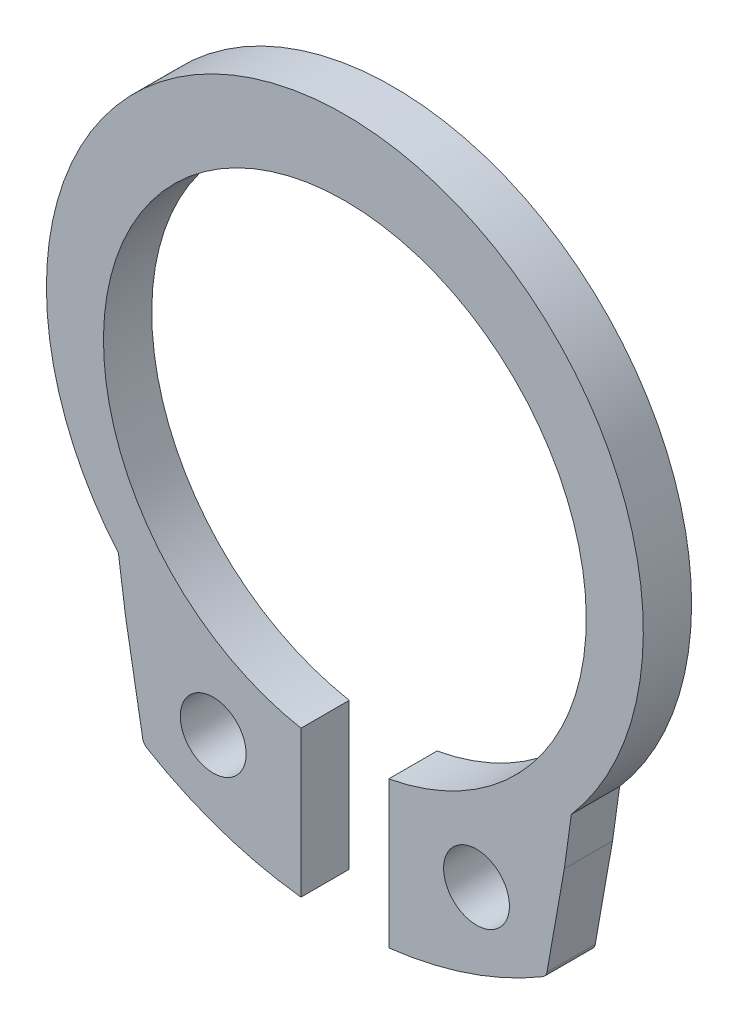
from build123d import *

# Parameters (mm, degrees)
SKETCH1_R           = 0.75
BOSS_EXTRUDE1_DEPTH = 1.1


with BuildPart() as part:
    # Sketch1 → Boss-Extrude1 (new body)
    with BuildSketch(Plane.XY):
        with BuildLine():
            Line((1, -5.408326913), (1, -6.326068688))
            Line((1, -6.326068688), (1, -7.130217388))
            Line((1, -7.130217388), (1, -8.742997198))
            ThreePointArc((1, -8.742997198), (2.818656417, -8.336376671), (4.510908199, -7.555905454))
            ThreePointArc((4.510908199, -7.555905454), (4.573051873, -7.497695365), (4.605349108, -7.418909965))
            Line((4.605349108, -7.418909965), (5, -5.180733539))
            Line((5, -5.180733539), (5.160454845, -4.028284746))
            ThreePointArc((5.160454845, -4.028284746), (0, 7.2), (-5.160454845, -4.028284746))
            Line((-5.160454845, -4.028284746), (-5, -5.180733539))
            Line((-5, -5.180733539), (-4.605349108, -7.418909965))
            ThreePointArc((-4.605349108, -7.418909965), (-4.573051873, -7.497695365), (-4.510908199, -7.555905454))
            ThreePointArc((-4.510908199, -7.555905454), (-2.818656417, -8.336376671), (-1, -8.742997198))
            Line((-1, -8.742997198), (-1, -7.130217388))
            Line((-1, -7.130217388), (-1, -5.408326913))
            ThreePointArc((-1, -5.408326913), (0, 5.5), (1, -5.408326913))
        make_face()
        with Locations((-3, -6.545227269)):
            Circle(SKETCH1_R, mode=Mode.SUBTRACT)
        with Locations((3, -6.545227269)):
            Circle(SKETCH1_R, mode=Mode.SUBTRACT)
    extrude(amount=BOSS_EXTRUDE1_DEPTH)


solid = part.part
